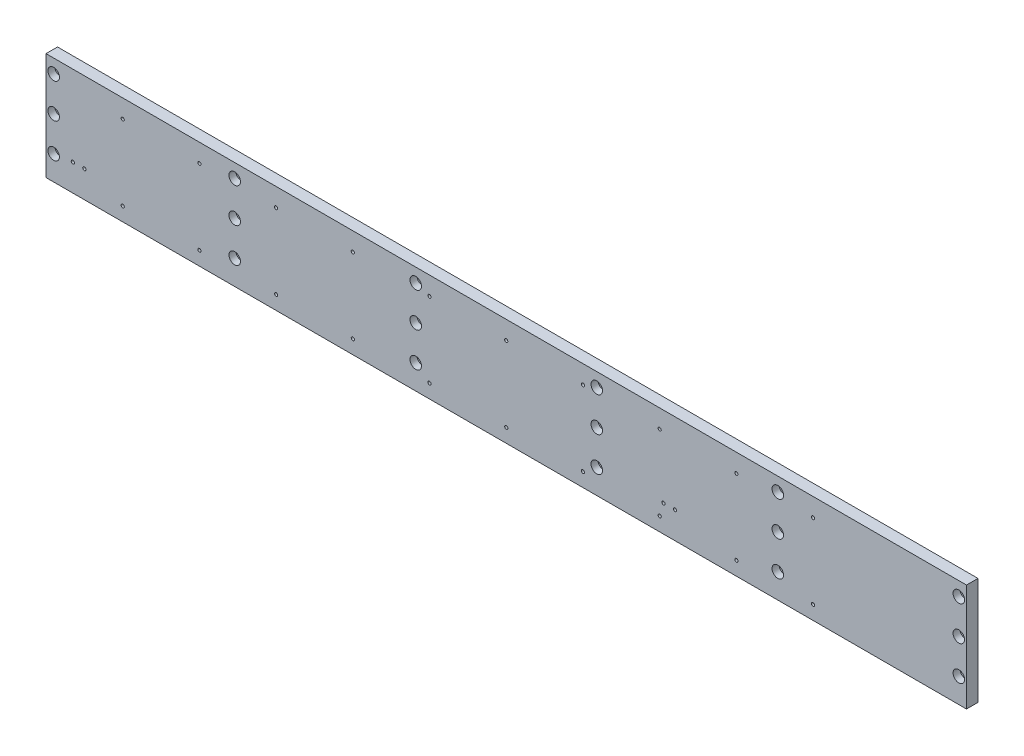
from build123d import *

# Parameters (mm, degrees)
SKETCH_1_W                = 1200
SKETCH_1_H                = 140
EXTRUDE_1_DEPTH           = 7.5
PATTERN_LINEAR_1_COUNT    = 6
PATTERN_LINEAR_1_PITCH    = 236
HOLE_WIZARD_1_D           = 9
HOLE_WIZARD_1_CBORE_D     = 15
HOLE_WIZARD_1_CBORE_DEPTH = 9
PATTERN_LINEAR_2_COUNT    = 6
PATTERN_LINEAR_2_PITCH    = 236
HOLE_WIZARD_M5_1_D        = 4.2
PATTERN_LINEAR_3_COUNT    = 2
PATTERN_LINEAR_3_PITCH    = 770
HOLE_WIZARD_M5_2_D        = 4.2
PATTERN_LINEAR_4_COUNT    = 10
PATTERN_LINEAR_4_PITCH    = 100


with BuildPart() as part:
    # 草图1 → 凸台-拉伸1 (new, symmetric)
    with BuildSketch(Plane.XY):
        Rectangle(SKETCH_1_W, SKETCH_1_H)
    extrude(amount=EXTRUDE_1_DEPTH, both=True)

    # 草图3 → M6 螺纹孔1 (revolve, cut)
    with BuildSketch(Plane(origin=(-590, -70, 0), x_dir=(0, 0, -1), z_dir=(1, 0, 0))):
        Polygon((0, 0), (0, 20.002151548), (2.5, 18.5), (2.5, 0), align=None)
    hole_wizard_m6_1 = revolve(axis=Axis((-590, -76.35, 0), (0, 1, 0)), mode=Mode.SUBTRACT)

    # 阵列(线性)1: M6 螺纹孔1 ×6
    with Locations(*[(i * PATTERN_LINEAR_1_PITCH, 0, 0) for i in range(1, PATTERN_LINEAR_1_COUNT)]):
        add(hole_wizard_m6_1, mode=Mode.SUBTRACT)

    # 打孔尺寸(%根据)内六角圆柱头螺钉的类型1 (through all)
    with Locations(Plane.XY.offset(7.5)):
        with Locations((-590, 52), (-590, 7), (-590, -38)):
            hole_wizard_1 = CounterBoreHole(HOLE_WIZARD_1_D / 2, HOLE_WIZARD_1_CBORE_D / 2, HOLE_WIZARD_1_CBORE_DEPTH)

    # 阵列(线性)2: 打孔尺寸(%根据)内六角圆柱头螺钉的类型1 ×6
    with Locations(*[(i * PATTERN_LINEAR_2_PITCH, 0, 0) for i in range(1, PATTERN_LINEAR_2_COUNT)]):
        add(hole_wizard_1, mode=Mode.SUBTRACT)

    # M5 螺纹孔1 (through all)
    with Locations(Plane(origin=(0, 0, -7.5), x_dir=(-1, 0, 0), z_dir=(0, 0, -1))):
        with Locations((550, -35), (565, -35)):
            hole_wizard_m5_1 = Hole(HOLE_WIZARD_M5_1_D / 2)

    # 阵列(线性)3: M5 螺纹孔1 ×2
    with Locations(*[(i * PATTERN_LINEAR_3_PITCH, 0, 0) for i in range(1, PATTERN_LINEAR_3_COUNT)]):
        add(hole_wizard_m5_1, mode=Mode.SUBTRACT)

    # M5 螺纹孔2 (through all)
    with Locations(Plane.XY.offset(7.5)):
        with Locations((-500, 46), (-500, -52)):
            hole_wizard_m5_2 = Hole(HOLE_WIZARD_M5_2_D / 2)

    # 阵列(线性)4: M5 螺纹孔2 ×10
    with Locations(*[(i * PATTERN_LINEAR_4_PITCH, 0, 0) for i in range(1, PATTERN_LINEAR_4_COUNT)]):
        add(hole_wizard_m5_2, mode=Mode.SUBTRACT)


solid = part.part
